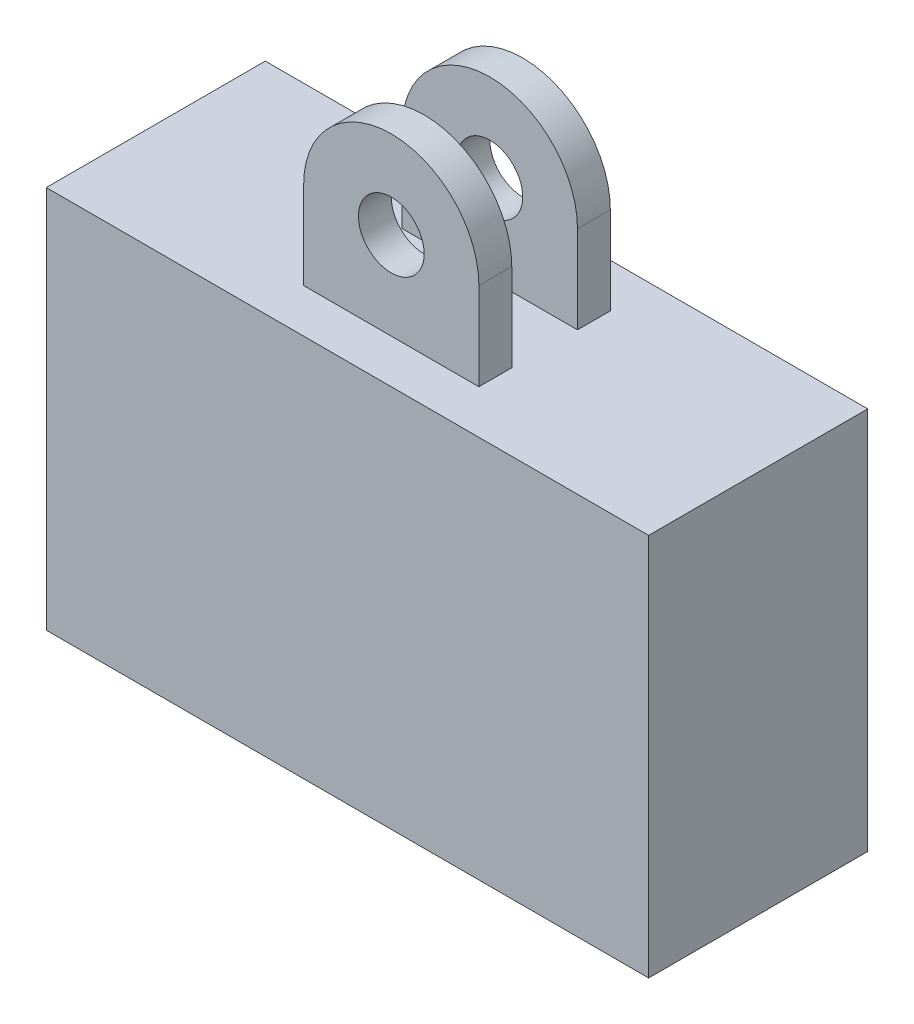
SolidWorks part; units mm, degrees
ref_plane "Front Plane" through (0, 0, 0) normal (0, 0, 1) x (1, 0, 0)
ref_plane "Top Plane" through (0, 0, 0) normal (0, 1, 0) x (1, 0, 0)
ref_plane "Right Plane" through (0, 0, 0) normal (1, 0, 0) x (0, 0, -1)
other "Configuration Table"
sketch "Sketch1" plane through (0, 0, 0) normal (0, 0, 1) x (1, 0, 0)
  line L1 (-27.5, 17.5) -> (27.5, 17.5)
  line L2 (-27.5, 17.5) -> (-27.5, -17.5)
  line L3 (-27.5, -17.5) -> (27.5, -17.5)
  line L4 (27.5, 17.5) -> (27.5, -17.5)
  line L5 (-27.5, 17.5) -> (27.5, -17.5) construction
  line L6 (-27.5, -17.5) -> (27.5, 17.5) construction
  point P0 (0, 0)
  dimension "D1" = 55
  dimension "D2" = 35
extrude "Boss-Extrude1" add sketch "Sketch1" along normal blind 20
sketch "Sketch2" plane through (0, 17.5, 0) normal (0, 1, 0) x (1, 0, 0)
  line L0 (-27.5, -10) -> (27.5, -10) construction
  line L1 (-8, -4) -> (8, -4)
  line L2 (-8, -4) -> (-8, -16)
  line L3 (-8, -16) -> (8, -16)
  line L4 (8, -4) -> (8, -16)
  line L5 (-8, -4) -> (8, -16) construction
  line L6 (-8, -16) -> (8, -4) construction
  line L7 (-27.5, -20) -> (-27.5, 0) construction
  line L8 (27.5, -20) -> (27.5, 0) construction
  point P0 (0, -10)
  dimension "D1" = 12
  dimension "D2" = 16
  dimension "D3" = 6
extrude "Boss-Extrude2" add sketch "Sketch2" along normal blind 16
sketch "Sketch3" plane through (0, 33.5, 0) normal (0, 1, 0) x (1, 0, 0)
  line L0 (8, -16) -> (8, -4) construction
  line L1 (-8, -7) -> (8, -7)
  line L2 (-8, -7) -> (-8, -13)
  line L3 (-8, -13) -> (8, -13)
  line L4 (8, -7) -> (8, -13)
  line L5 (-8, -7) -> (8, -13) construction
  line L6 (-8, -13) -> (8, -7) construction
  line L7 (8, -4) -> (-8, -4) construction
  point P0 (0, -10)
  dimension "D1" = 6
  dimension "D2" = 16
  dimension "D3" = 3
extrude "Cut-Extrude1" cut sketch "Sketch3" against normal blind 16 and the other way through all
sketch "Sketch4" plane through (0, 0, 16) normal (0, 0, 1) x (1, 0, 0)
  line L0 (-8, 33.5) -> (8, 33.5) construction
  line L1 (-8, 25.5) -> (-21.6447, 27.6903)
  line L2 (-21.6447, 27.6903) -> (-8, 39.0362)
  line L3 (-8, 39.0362) -> (25.7488, 31.9899)
  line L4 (25.7488, 31.9899) -> (8, 25.5)
  line L5 (8, 33.5) -> (8, 17.5) construction
  arc A0 (8, 25.5) -> (-8, 25.5) centre (0, 25.5) ccw
  circle A1 centre (0, 25.5) radius 3
  dimension "D1" = 6
extrude "Cut-Extrude2" cut sketch "Sketch4" against normal through all
